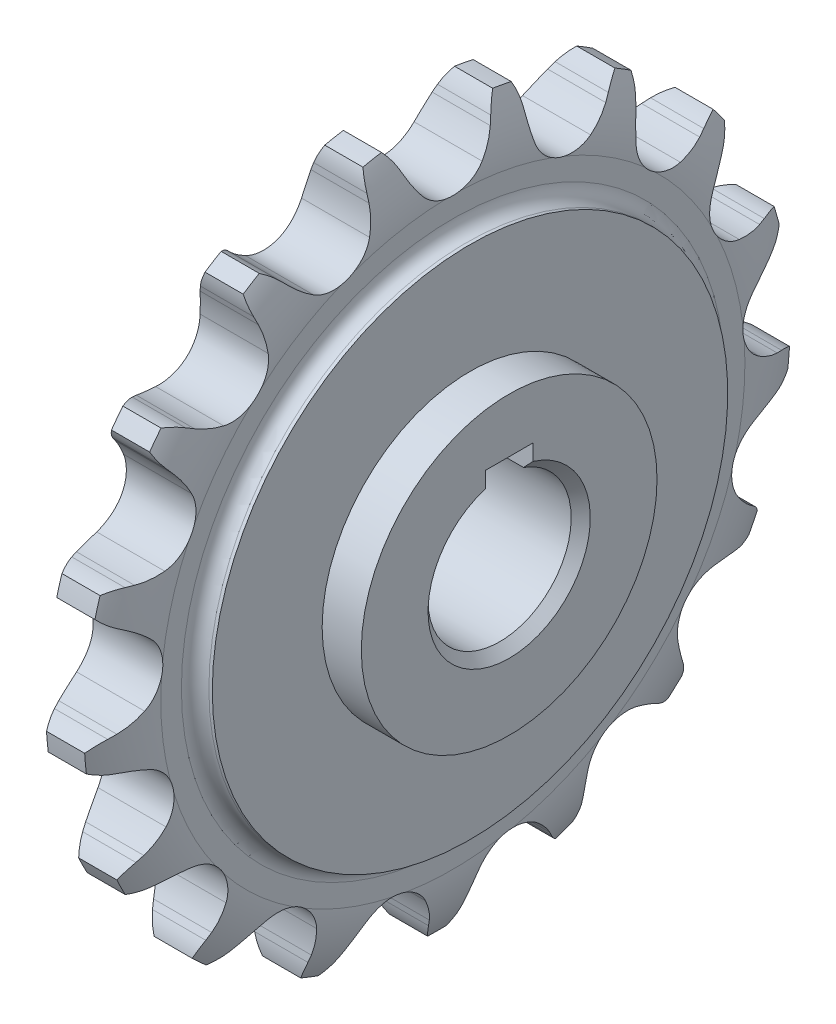
from build123d import *

# Parameters (mm, degrees)
CUT_EXTRUDE_1_DEPTH      = 5.449206907
PATTERN_CIRCULAR_1_COUNT = 17
SKETCH_3_W               = 4.101586186
SKETCH_3_H               = 7.991158276
SKETCH_4_W               = 5
SKETCH_4_H               = 2.72893214
CUT_EXTRUDE_2_DEPTH      = 55.379316976
CHAMFER_1_SIZE           = 1
CHAMFER_3_SIZE           = 1


with BuildPart() as part:
    # 草图1 → 旋转1 (revolve)
    with BuildSketch(Plane.XY, mode=Mode.PRIVATE) as revolve_1_sk:
        with BuildLine():
            Line((-5.449206907, 7.5), (-5.449206907, 27))
            Line((-5.449206907, 27), (-5.089415525, 27))
            ThreePointArc((-5.089415525, 27), (-4.071771823, 27.421521823), (-3.65025, 28.439165525))
            Line((-3.65025, 28.439165525), (-3.65025, 30.597913814))
            ThreePointArc((-3.65025, 30.597913814), (-3.248667458, 33.908278728), (-1.99925, 37))
            Line((-1.99925, 37), (1.99925, 37))
            ThreePointArc((1.99925, 37), (3.248667458, 33.908278728), (3.65025, 30.597913814))
            Line((3.65025, 30.597913814), (3.65025, 28.439165525))
            ThreePointArc((3.65025, 28.439165525), (4.071771823, 27.421521823), (5.089415525, 27))
            Line((5.089415525, 27), (5.449206907, 27))
            Line((5.449206907, 27), (5.449206907, 7.5))
            Line((5.449206907, 7.5), (-5.449206907, 7.5))
        make_face()
    revolve(revolve_1_sk.sketch.rotate(Axis((-6.35, 0, 0), (1, 0, 0)), 90), axis=Axis((-6.35, 0, 0), (1, 0, 0)))

    # 草图2 → 切除-拉伸1 (cut, symmetric)
    with BuildSketch(Plane(origin=(0, 0, 0), x_dir=(0, 0, -1), z_dir=(1, 0, 0))):
        with BuildLine():
            Line((4.525990365, 34.317747091), (4.828460685, 35.00277706))
            ThreePointArc((4.828460685, 35.00277706), (5.264672951, 35.810417906), (5.823136285, 36.538898229))
            ThreePointArc((5.823136285, 36.538898229), (0, 37), (-5.823136285, 36.538898229))
            ThreePointArc((-5.823136285, 36.538898229), (-5.264672951, 35.810417906), (-4.828460685, 35.00277706))
            Line((-4.828460685, 35.00277706), (-4.525990365, 34.317747091))
            ThreePointArc((-4.525990365, 34.317747091), (-3.912159361, 33.138588704), (-3.152466185, 32.047685738))
            ThreePointArc((-3.152466185, 32.047685738), (0, 30.528113814), (3.152466185, 32.047685738))
            ThreePointArc((3.152466185, 32.047685738), (3.912159361, 33.138588704), (4.525990365, 34.317747091))
        make_face()
    cut_extrude_1 = extrude(amount=CUT_EXTRUDE_1_DEPTH, both=True, mode=Mode.SUBTRACT)

    # 阵列(圆周)1: 切除-拉伸1 ×17 about axis
    pattern_circular_1_axis = Axis((0, 0, 0), (1, 0, 0))
    for i in range(1, PATTERN_CIRCULAR_1_COUNT):
        add(cut_extrude_1.rotate(pattern_circular_1_axis, i * 360 / PATTERN_CIRCULAR_1_COUNT), mode=Mode.SUBTRACT)

    # 草图3 → 旋转2 (revolve)
    with BuildSketch(Plane.XY, mode=Mode.PRIVATE) as revolve_2_sk:
        with Locations((7.5, 11.495579138)):
            Rectangle(SKETCH_3_W, SKETCH_3_H)
    revolve(revolve_2_sk.sketch.rotate(Axis((0, 0, 0), (1, 0, 0)), 90), axis=Axis((0, 0, 0), (1, 0, 0)))

    # 草图4 → 切除-拉伸2 (cut, through all)
    with BuildSketch(Plane.ZY.offset(5.449206907)):
        with Locations((0, 8.435533882)):
            Rectangle(SKETCH_4_W, SKETCH_4_H)
    extrude(amount=-CUT_EXTRUDE_2_DEPTH, mode=Mode.SUBTRACT)

    # 倒角1
    chamfer_1_edges = [part.edges().sort_by_distance(p)[0] for p in [
        (-5.449206907, -7.5, 0),
    ]]
    chamfer(chamfer_1_edges, length=CHAMFER_1_SIZE)

    # 倒角3
    chamfer_3_edges = [part.edges().sort_by_distance(p)[0] for p in [
        (9.550793093, -7.5, 0),
    ]]
    chamfer(chamfer_3_edges, length=CHAMFER_3_SIZE)


solid = part.part
